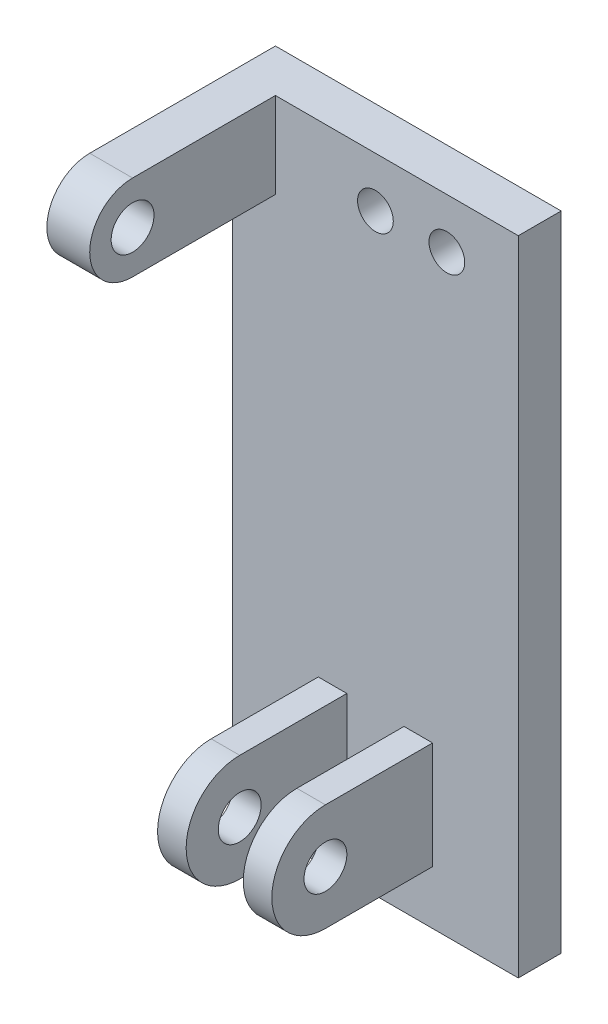
from build123d import *

# Parameters (mm, degrees)
SKETCH1_W           = 40
SKETCH1_H           = 90
BOSS_EXTRUDE1_DEPTH = 6
SKETCH2_R           = 2.5
CUT_EXTRUDE1_DEPTH  = 6
SKETCH3_R           = 3
BOSS_EXTRUDE2_DEPTH = 6
BOSS_EXTRUDE3_START = 4
SKETCH4_R           = 3
BOSS_EXTRUDE3_DEPTH = 4


with BuildPart() as part:
    # Sketch1 → Boss-Extrude1 (new body)
    with BuildSketch(Plane.XY):
        Rectangle(SKETCH1_W, SKETCH1_H)
    extrude(amount=BOSS_EXTRUDE1_DEPTH)

    # Sketch2 → Cut-Extrude1 (cut)
    with BuildSketch(Plane.XY.offset(6)):
        with Locations((0, 38)):
            Circle(SKETCH2_R)
        with Locations((10, 38)):
            Circle(SKETCH2_R)
    extrude(amount=-CUT_EXTRUDE1_DEPTH, mode=Mode.SUBTRACT)

    # Sketch3 → Boss-Extrude2 (add)
    with BuildSketch(Plane.ZY.offset(20)):
        with BuildLine():
            Line((26, 45), (6, 45))
            Line((6, 45), (6, 33))
            Line((6, 33), (26, 33))
            ThreePointArc((26, 33), (32, 39), (26, 45))
        make_face()
        with Locations(Location((26, 39, 0), (0, 0, 270))):
            Circle(SKETCH3_R, mode=Mode.SUBTRACT)
    extrude(amount=-BOSS_EXTRUDE2_DEPTH)

    # Sketch4 → Boss-Extrude3 (add)
    with BuildSketch(Plane(origin=(0, 0, 0), x_dir=(0, 0, -1), z_dir=(1, 0, 0)).offset(BOSS_EXTRUDE3_START)):
        with BuildLine():
            Line((-21, -22.5), (-6, -22.5))
            Line((-6, -22.5), (-6, -37.5))
            Line((-6, -37.5), (-21, -37.5))
            ThreePointArc((-21, -37.5), (-28.5, -30), (-21, -22.5))
        make_face()
        with Locations((-21, -30)):
            Circle(SKETCH4_R, mode=Mode.SUBTRACT)
    boss_extrude3 = extrude(amount=BOSS_EXTRUDE3_DEPTH)

    # Mirror1: Boss-Extrude3 across plane
    add(boss_extrude3.mirror(Plane(origin=(0, 0, 0), x_dir=(0, 0, 1), z_dir=(1, 0, 0))))


solid = part.part
